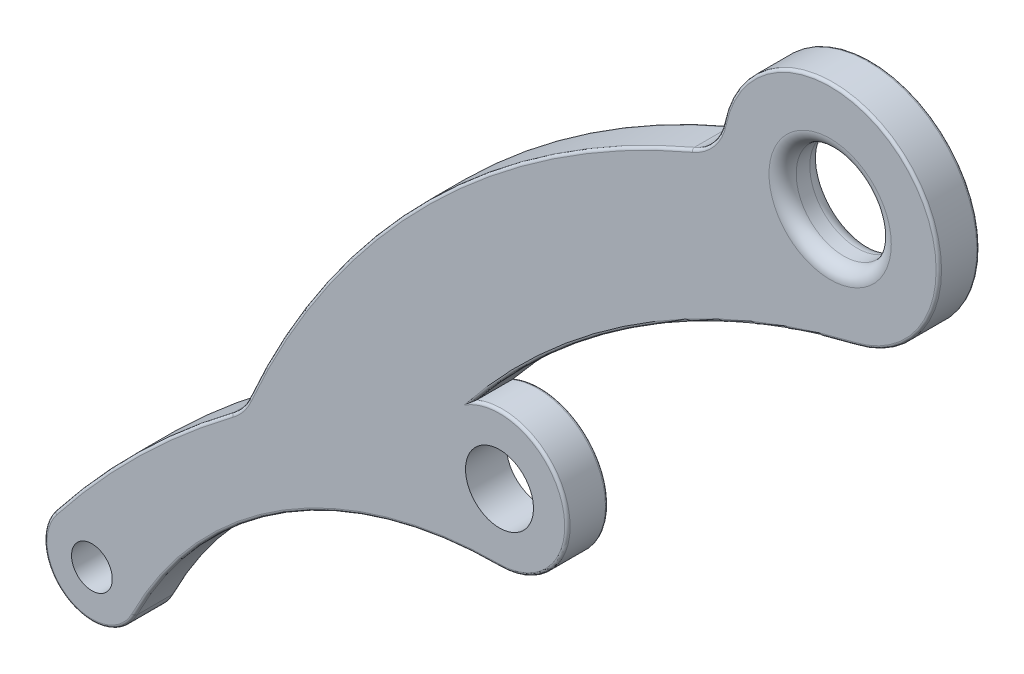
SolidWorks part; units mm, degrees
ref_plane "Front Plane" through (0, 0, 0) normal (0, 0, 1) x (1, 0, 0)
ref_plane "Top Plane" through (0, 0, 0) normal (0, 1, 0) x (1, 0, 0)
ref_plane "Right Plane" through (0, 0, 0) normal (1, 0, 0) x (0, 0, -1)
other "Configuration Table"
ref_plane "Plane1" through (0, 0, 15) normal (0, 0, 1) x (1, 0, 0)
sketch "Sketch1" plane through (0, 0, 15) normal (0, 0, 1) x (1, 0, 0)
  arc A0 (231.7369, 248.1227) -> (55.6554, 77.7522) centre (341.7108, -41.7147) ccw
  arc A1 (55.6554, 77.7522) -> (-13.7676, 10.8029) centre (261.5848, -205.255) ccw
  arc A2 (-13.7676, 10.8029) -> (15.6477, -7.8358) centre (0, 0) ccw
  arc A3 (15.6477, -7.8358) -> (149.9672, 75) centre (149.7707, -74.9998) cw
  arc A4 (149.9672, 75) -> (140.7152, 123.2119) centre (150, 100) ccw
  arc A5 (140.7152, 123.2119) -> (281.0285, 211.1047) centre (341.7108, -41.7147) cw
  arc A6 (281.0285, 211.1047) -> (231.7369, 248.1227) centre (271.6928, 250) ccw
extrude "Boss-Extrude1" add sketch "Sketch1" against normal blind 15
hole_wizard "M30 Clearance Hole1" positions "Sketch3" profile "Sketch2" hole size "M30" standard "ANSI Metric"
sketch "Sketch3" plane through (0, 0, 0) normal (0, 0, -1) x (-1, 0, 0)
  point P0 (-271.6928, 250)
sketch "Sketch2" plane through (271.6928, 250, 0) normal (1, 0, 0) x (0, 1, 0)
  line L0 (0, 0) -> (0, 15)
  line L1 (0, 15) -> (17.5, 15)
  line L2 (17.5, 15) -> (17.5, 0)
  line L5 (17.5, 0) -> (0, 0)
  line L11 (0, -6.35) -> (0, 107.95) construction
  dimension "通孔孔直径" = 35
  dimension "通孔孔深度" = 15
hole_wizard "Ø25.0 (25) Diameter Hole1" positions "Sketch5" profile "Sketch4" hole size "Ø25.0" standard "ANSI Metric"
sketch "Sketch5" plane through (0, 0, 0) normal (0, 0, -1) x (-1, 0, 0)
  point P0 (-150, 100)
sketch "Sketch4" plane through (150, 100, 0) normal (1, 0, 0) x (0, 1, 0)
  line L0 (0, 0) -> (0, 15)
  line L1 (0, 15) -> (12.5, 15)
  line L2 (12.5, 15) -> (12.5, 0)
  line L5 (12.5, 0) -> (0, 0)
  line L11 (0, -6.35) -> (0, 107.95) construction
  dimension "通孔孔直径" = 25
  dimension "通孔孔深度" = 15
hole_wizard "Ø15.0 (15) Diameter Hole1" positions "Sketch7" profile "Sketch6" hole size "Ø15.0" standard "ANSI Metric"
sketch "Sketch7" plane through (0, 0, 0) normal (0, 0, -1) x (-1, 0, 0)
  point P0 (0, 0)
sketch "Sketch6" plane through (0, 0, 0) normal (1, 0, 0) x (0, 1, 0)
  line L0 (0, 0) -> (0, 15)
  line L1 (0, 15) -> (7.5, 15)
  line L2 (7.5, 15) -> (7.5, 0)
  line L5 (7.5, 0) -> (0, 0)
  line L11 (0, -6.35) -> (0, 107.95) construction
  dimension "通孔孔直径" = 15
  dimension "通孔孔深度" = 15
fillet "Fillet1" radius 20 2 edges at (231.7369, 248.1227, 7.5) (55.6554, 77.7522, 7.5)
fillet "Fillet2" radius 1 18 edges at (203.6887, 178.6257, 0) (299.5185, 278.7355, 0) (228.3971, 249.4408, 0) (123.7919, 178.7652, 0) (55.0826, 78.1935, 0) (16.7342, 44.8413, 0) (-9.3666, -14.7823, 0) (71.0337, 52.6735, 0) (174.552, 104.7116, 0) (203.6887, 178.6257, 15) (174.552, 104.7116, 15) (299.5185, 278.7355, 15) (71.0337, 52.6735, 15) (228.3971, 249.4408, 15) (-9.3666, -14.7823, 15) (123.7919, 178.7652, 15) (16.7342, 44.8413, 15) (55.0826, 78.1935, 15)
fillet "Fillet3" radius 5 2 edges at (254.1928, 250, 15) (254.1928, 250, 0)
